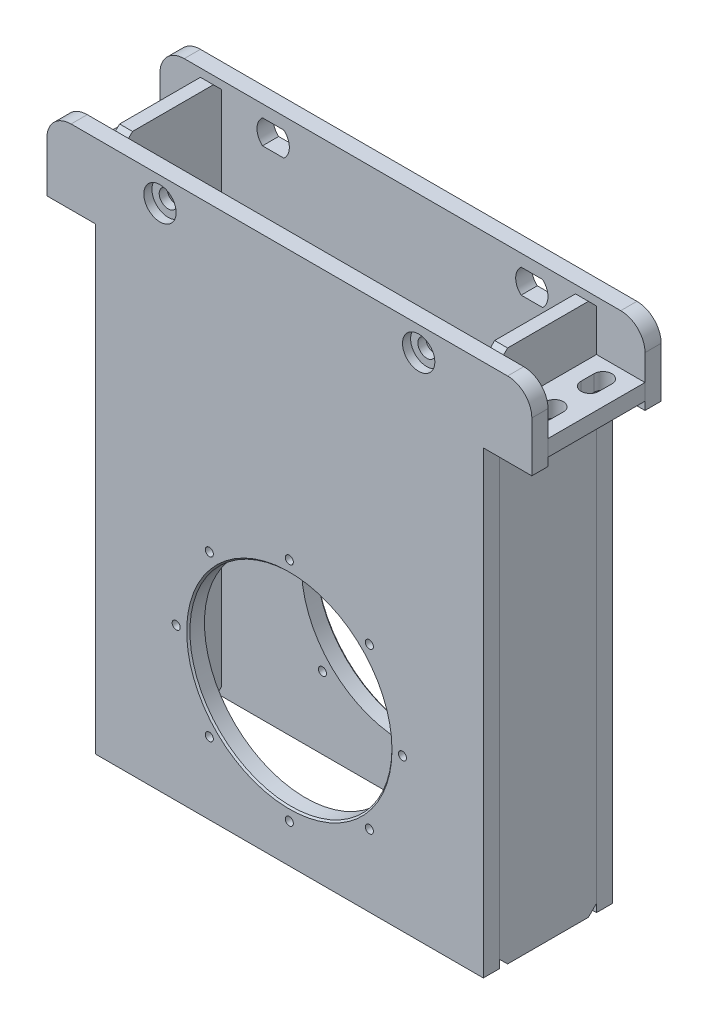
from build123d import *

# Parameters (mm, degrees)
SKETCH1_W             = 300
SKETCH1_H             = 330
BOSS_EXTRUDE1_DEPTH   = 10
SKETCH2_R             = 7.5
CUT_EXTRUDE1_DEPTH    = 10
LPATTERN1_COUNT       = 2
LPATTERN1_PITCH       = 160
SKETCH12_W            = 8
SKETCH12_H            = 330
BOSS_EXTRUDE2_DEPTH   = 60
BOSS_EXTRUDE2_2_DEPTH = 60
SKETCH13_R            = 7.5
BOSS_EXTRUDE3_DEPTH   = 10
SKETCH14_W            = 60
SKETCH14_H            = 10
BOSS_EXTRUDE4_DEPTH   = 30
CUT_EXTRUDE6_DEPTH    = 10
FILLET1_R             = 15
SKETCH3_R             = 62.5
CUT_EXTRUDE2_DEPTH    = 170
CIRPATTERN1_COUNT     = 8
SKETCH16_W            = 30
SKETCH16_H            = 284
CUT_EXTRUDE3_DEPTH    = 141
CIRPATTERN2_COUNT     = 8
SKETCH21_R            = 10
CUT_EXTRUDE4_DEPTH    = 18
LPATTERN2_COUNT       = 2
LPATTERN2_PITCH       = 160
CUT_EXTRUDE5_START    = -5
SKETCH22_R            = 10
CUT_EXTRUDE5_DEPTH    = 5
CHAMFER1_SIZE         = 1
CHAMFER2_SIZE         = 1
SKETCH23_R            = 7.5
SKETCH23_R_2          = 5.5
BOSS_EXTRUDE5_DEPTH   = 5
BOSS_EXTRUDE6_DEPTH   = 10
CHAMFER3_SIZE         = 5
CHAMFER4_SIZE         = 5


with BuildPart() as part:
    # Sketch1 → Boss-Extrude1 (new body)
    with BuildSketch(Plane.XY):
        Rectangle(SKETCH1_W, SKETCH1_H)
    extrude(amount=BOSS_EXTRUDE1_DEPTH)

    # Sketch2 → Cut-Extrude1 (cut)
    with BuildSketch(Plane.XY.offset(10)):
        with Locations((-80, 150)):
            Circle(SKETCH2_R)
    cut_extrude1 = extrude(amount=-CUT_EXTRUDE1_DEPTH, mode=Mode.SUBTRACT)

    # LPattern1: Cut-Extrude1 ×2
    with Locations(*[(i * LPATTERN1_PITCH, 0, 0) for i in range(1, LPATTERN1_COUNT)]):
        add(cut_extrude1, mode=Mode.SUBTRACT)

    # Fillet1
    fillet1_edges = [part.edges().sort_by_distance(p)[0] for p in [
        (-150, 165, 5),
        (150, 165, 5),
    ]]
    fillet(fillet1_edges, radius=FILLET1_R)


with BuildPart() as body_2:
    # Sketch12 → Boss-Extrude2 (new body)
    with BuildSketch(Plane.XY.offset(10)):
        with Locations((116, 0)):
            Rectangle(SKETCH12_W, SKETCH12_H)
    extrude(amount=BOSS_EXTRUDE2_DEPTH)

    # Chamfer4
    chamfer4_edges = [body_2.edges().sort_by_distance(p)[0] for p in [
        (116, -165, 70),
        (116, -165, 10),
        (116, 165, 10),
        (116, 165, 70),
    ]]
    chamfer(chamfer4_edges, length=CHAMFER4_SIZE)


with BuildPart() as body_3:
    # Sketch12 → Boss-Extrude2 2 (new body)
    with BuildSketch(Plane.XY.offset(10)):
        with Locations((-116, 0)):
            Rectangle(SKETCH12_W, SKETCH12_H)
    extrude(amount=BOSS_EXTRUDE2_2_DEPTH)

    # Chamfer3
    chamfer3_edges = [body_3.edges().sort_by_distance(p)[0] for p in [
        (-116, 165, 70),
        (-116, 165, 10),
        (-116, -165, 10),
        (-116, -165, 70),
    ]]
    chamfer(chamfer3_edges, length=CHAMFER3_SIZE)


with BuildPart() as body_4:
    # Sketch13 → Boss-Extrude3 (new body)
    with BuildSketch(Plane.XY.offset(70)):
        with BuildLine():
            Line((150, -165), (-150, -165))
            Line((-150, -165), (-150, 150))
            ThreePointArc((-150, 150), (-145.606601718, 160.606601718), (-135, 165))
            Line((-135, 165), (135, 165))
            ThreePointArc((135, 165), (145.606601718, 160.606601718), (150, 150))
            Line((150, 150), (150, -165))
        make_face()
        with Locations((80, 150)):
            Circle(SKETCH13_R, mode=Mode.SUBTRACT)
        with Locations((-80, 150)):
            Circle(SKETCH13_R, mode=Mode.SUBTRACT)
    extrude(amount=BOSS_EXTRUDE3_DEPTH)


with BuildPart() as body_5:
    # Sketch14 → Boss-Extrude4 (new body)
    with BuildSketch(Plane(origin=(120, 0, 0), x_dir=(0, 0, -1), z_dir=(1, 0, 0))):
        with Locations((-40, 129)):
            Rectangle(SKETCH14_W, SKETCH14_H)
    extrude(amount=BOSS_EXTRUDE4_DEPTH)

    # Sketch26 → Cut-Extrude6 (cut)
    with BuildSketch(Plane(origin=(0, 134, 0), x_dir=(1, 0, 0), z_dir=(0, 1, 0))):
        with BuildLine():
            Line((140.5, -21), (140.5, -29))
            ThreePointArc((140.5, -29), (135, -34.5), (129.5, -29))
            Line((129.5, -29), (129.5, -21))
            ThreePointArc((129.5, -21), (135, -15.5), (140.5, -21))
        make_face()
        with BuildLine():
            Line((129.5, -59), (129.5, -51))
            ThreePointArc((129.5, -51), (135, -45.5), (140.5, -51))
            Line((140.5, -51), (140.5, -59))
            ThreePointArc((140.5, -59), (135, -64.5), (129.5, -59))
        make_face()
    extrude(amount=-CUT_EXTRUDE6_DEPTH, mode=Mode.SUBTRACT)


with BuildPart() as body_6:
    # Mirror1: mirrored copy
    add(body_5.part.mirror(Plane(origin=(0, 0, 0), x_dir=(0, 0, 1), z_dir=(1, 0, 0))))


with BuildPart() as cut_extrude2_tool:
    # Sketch3 → Cut-Extrude2 (new body)
    with BuildSketch(Plane.XY):
        with Locations((0, -71)):
            Circle(SKETCH3_R)
    extrude(amount=CUT_EXTRUDE2_DEPTH)


with BuildPart() as part_1:
    add(part.part)

    # Cut-Extrude2: cut by cut_extrude2_tool
    add(cut_extrude2_tool.part, mode=Mode.SUBTRACT)

    # Sketch5 → M6 Tapped Hole1 (revolve, cut)
    with BuildSketch(Plane(origin=(49.497474683, -21.502525317, 10), x_dir=(0, -1, 0), z_dir=(1, 0, 0))):
        Polygon((0, 0), (0, 18.502151548), (2.5, 17), (2.5, 0), align=None)
    m6_tapped_hole1 = revolve(axis=Axis((49.497474683, -21.502525317, 16.35), (0, 0, -1)), mode=Mode.SUBTRACT)

    # CirPattern1: M6 Tapped Hole1 ×8 about axis
    cirpattern1_axis = Axis((0, -71, 0), (0, 0, 1))
    for i in range(1, CIRPATTERN1_COUNT):
        add(m6_tapped_hole1.rotate(cirpattern1_axis, i * 360 / CIRPATTERN1_COUNT), mode=Mode.SUBTRACT)


with BuildPart() as body_4_1:
    add(body_4.part)

    # Cut-Extrude2: cut by cut_extrude2_tool
    add(cut_extrude2_tool.part, mode=Mode.SUBTRACT)


with BuildPart() as cut_extrude3_tool:
    # Sketch16 → Cut-Extrude3 (new body)
    with BuildSketch(Plane.XY.offset(80)):
        with Locations((135, -23)):
            Rectangle(SKETCH16_W, SKETCH16_H)
        with Locations((-135, -23)):
            Rectangle(SKETCH16_W, SKETCH16_H)
    extrude(amount=-CUT_EXTRUDE3_DEPTH)


with BuildPart() as part_2:
    add(part_1.part)

    # Cut-Extrude3: cut by cut_extrude3_tool
    add(cut_extrude3_tool.part, mode=Mode.SUBTRACT)

    # Sketch21 → Cut-Extrude4 (cut)
    with BuildSketch(Plane(origin=(0, 0, 0), x_dir=(-1, 0, 0), z_dir=(0, 0, -1))):
        with Locations((-80, 150)):
            Circle(SKETCH21_R)
    cut_extrude4 = extrude(amount=-CUT_EXTRUDE4_DEPTH, mode=Mode.SUBTRACT)

    # LPattern2: Cut-Extrude4 ×2
    with Locations(*[(-i * LPATTERN2_PITCH, 0, 0) for i in range(1, LPATTERN2_COUNT)]):
        add(cut_extrude4, mode=Mode.SUBTRACT)

    # Chamfer2
    chamfer2_edges = [part_2.edges().sort_by_distance(p)[0] for p in [
        (-62.5, -71, 0),
    ]]
    chamfer(chamfer2_edges, length=CHAMFER2_SIZE)

    # Sketch24 → Boss-Extrude6 (add)
    with BuildSketch(Plane(origin=(0, 0, 0), x_dir=(-1, 0, 0), z_dir=(0, 0, -1))):
        with BuildLine():
            ThreePointArc((86.614378278, 157.5), (80, 160), (73.385621722, 157.5))
            Line((73.385621722, 157.5), (86.614378278, 157.5))
        make_face()
        with BuildLine():
            Line((86.614378278, 142.5), (73.385621722, 142.5))
            ThreePointArc((73.385621722, 142.5), (80, 140), (86.614378278, 142.5))
        make_face()
        with BuildLine():
            ThreePointArc((-73.385621722, 157.5), (-80, 160), (-86.614378278, 157.5))
            Line((-86.614378278, 157.5), (-73.385621722, 157.5))
        make_face()
        with BuildLine():
            Line((-73.385621722, 142.5), (-86.614378278, 142.5))
            ThreePointArc((-86.614378278, 142.5), (-80, 140), (-73.385621722, 142.5))
        make_face()
    extrude(amount=-BOSS_EXTRUDE6_DEPTH)


with BuildPart() as body_4_2:
    add(body_4_1.part)

    # Cut-Extrude3: cut by cut_extrude3_tool
    add(cut_extrude3_tool.part, mode=Mode.SUBTRACT)

    # Sketch20 → M6 Tapped Hole2 (revolve, cut)
    with BuildSketch(Plane(origin=(-70, -71, 80), x_dir=(0, -1, 0), z_dir=(1, 0, 0))):
        Polygon((0, 0), (0, 26.002151548), (2.5, 24.5), (2.5, 0), align=None)
    m6_tapped_hole2 = revolve(axis=Axis((-70, -71, 86.35), (0, 0, -1)), mode=Mode.SUBTRACT)

    # CirPattern2: M6 Tapped Hole2 ×8 about axis
    cirpattern2_axis = Axis((0, -71, 0), (0, 0, 1))
    for i in range(1, CIRPATTERN2_COUNT):
        add(m6_tapped_hole2.rotate(cirpattern2_axis, i * 360 / CIRPATTERN2_COUNT), mode=Mode.SUBTRACT)

    # Sketch22 → Cut-Extrude5 (cut)
    with BuildSketch(Plane.XY.offset(80).offset(CUT_EXTRUDE5_START)):
        with Locations((80, 150)):
            Circle(SKETCH22_R)
        with Locations((-80, 150)):
            Circle(SKETCH22_R)
    extrude(amount=CUT_EXTRUDE5_DEPTH, mode=Mode.SUBTRACT)

    # Chamfer1
    chamfer1_edges = [body_4_2.edges().sort_by_distance(p)[0] for p in [
        (-62.5, -71, 80),
    ]]
    chamfer(chamfer1_edges, length=CHAMFER1_SIZE)

    # Sketch23 → Boss-Extrude5 (add)
    # profile 1 of 2: a face of its own
    with BuildSketch(Plane(origin=(0, 0, 70), x_dir=(-1, 0, 0), z_dir=(0, 0, -1))):
        with Locations((-80, 150)):
            Circle(SKETCH23_R)
        with Locations((-80, 150)):
            Circle(SKETCH23_R_2, mode=Mode.SUBTRACT)
    # profile 2 of 2: a face of its own
    with BuildSketch(Plane(origin=(0, 0, 70), x_dir=(-1, 0, 0), z_dir=(0, 0, -1))):
        with Locations((80, 150)):
            Circle(SKETCH23_R)
        with Locations((80, 150)):
            Circle(SKETCH23_R_2, mode=Mode.SUBTRACT)
    extrude(amount=-BOSS_EXTRUDE5_DEPTH)


solid = Compound([body_2.part, body_3.part, body_5.part, body_6.part, part_2.part, body_4_2.part])
